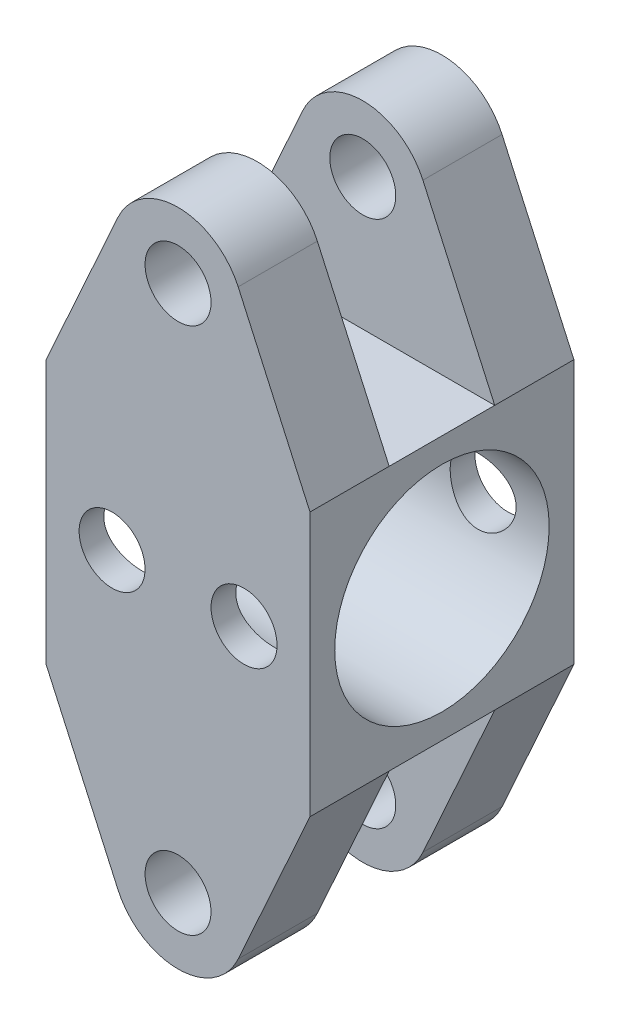
from build123d import *

# Parameters (mm, degrees)
SKETCH_1_R               = 5
EXTRUDE_1_DEPTH          = 20
CUT_EXTRUDE_1_DEPTH      = 58.445626465
CUT_EXTRUDE_1_DEPTH_BACK = 58.445626465
SKETCH_2_R               = 16.25
SKETCH_2_W               = 16
SKETCH_2_H               = 60


with BuildPart() as part:
    # 草图1 → 凸台-拉伸1 (new, symmetric)
    with BuildSketch(Plane.XY):
        with BuildLine():
            Line((20, -20), (20, 20))
            Line((20, 20), (9.114378278, 44.114378278))
            ThreePointArc((9.114378278, 44.114378278), (0, 50), (-9.114378278, 44.114378278))
            Line((-9.114378278, 44.114378278), (-20, 20))
            Line((-20, 20), (-20, -20))
            Line((-20, -20), (-9.114378278, -44.114378278))
            ThreePointArc((-9.114378278, -44.114378278), (0, -50), (9.114378278, -44.114378278))
            Line((9.114378278, -44.114378278), (20, -20))
        make_face()
        with Locations((0, 40)):
            Circle(SKETCH_1_R, mode=Mode.SUBTRACT)
        with Locations((10, 0)):
            Circle(SKETCH_1_R, mode=Mode.SUBTRACT)
        with Locations(Location((0, -40, 0), (0, 0, 180))):
            Circle(SKETCH_1_R, mode=Mode.SUBTRACT)
        with Locations(Location((-10, 0, 0), (0, 0, 180))):
            Circle(SKETCH_1_R, mode=Mode.SUBTRACT)
    extrude(amount=EXTRUDE_1_DEPTH, both=True)

    # 草图2 → 切除-拉伸1 (cut, two sides: drawn at the far end of the back side and taken through both)
    with BuildSketch(Plane(origin=(0, 0, 0), x_dir=(0, 0, -1), z_dir=(1, 0, 0)).offset(-CUT_EXTRUDE_1_DEPTH_BACK)):
        Circle(SKETCH_2_R)
        with Locations((0, 50)):
            Rectangle(SKETCH_2_W, SKETCH_2_H)
        with Locations((0, -50)):
            Rectangle(SKETCH_2_W, SKETCH_2_H)
    extrude(amount=CUT_EXTRUDE_1_DEPTH + CUT_EXTRUDE_1_DEPTH_BACK, mode=Mode.SUBTRACT)


solid = part.part
